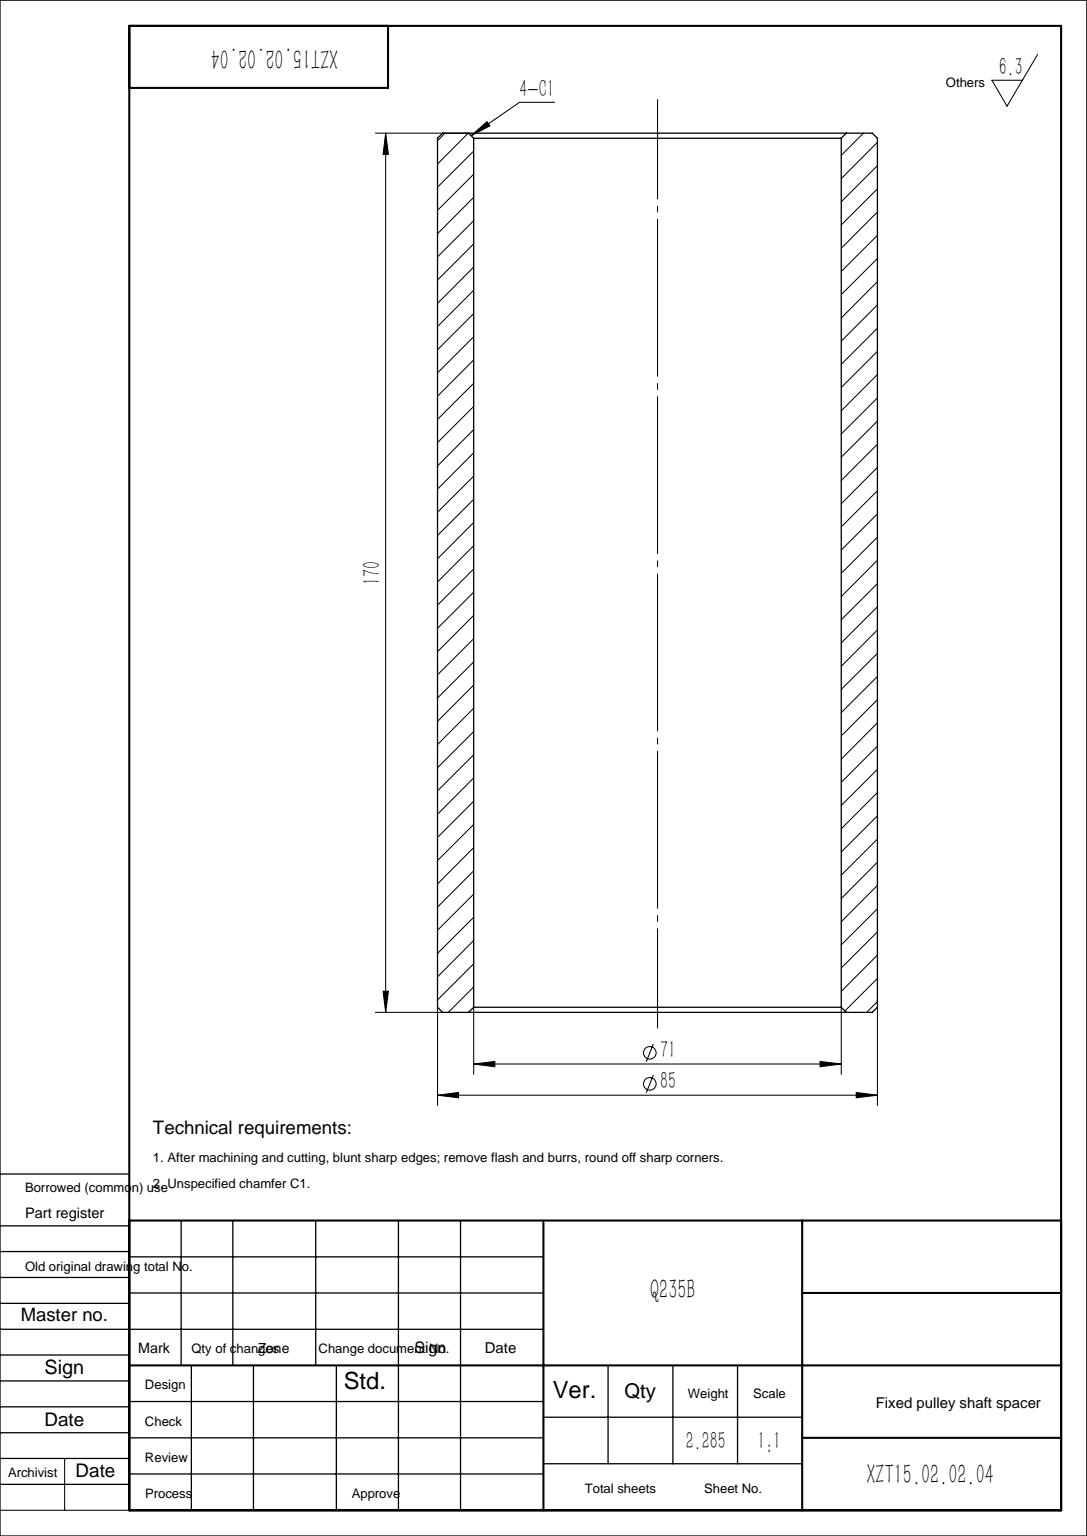
SolidWorks part; units mm, degrees
material "Q235B"
ref_plane "Front Plane" through (0, 0, 0) normal (0, 0, 1) x (1, 0, 0)
ref_plane "Top Plane" through (0, 0, 0) normal (0, 1, 0) x (1, 0, 0)
ref_plane "Right Plane" through (0, 0, 0) normal (1, 0, 0) x (0, 0, -1)
sketch "Sketch1" plane through (0, 0, 0) normal (0, 1, 0) x (1, 0, 0)
  circle A0 centre (0, 0) radius 35.5
  circle A1 centre (0, 0) radius 42.5
  dimension "D1" = 71
  dimension "D2" = 85
extrude "Boss-Extrude1" add sketch "Sketch1" along normal blind 170
chamfer "Chamfer2" distance 1 angle 45 4 edges at (0, 0, 35.5) (0, 170, 35.5) (0, 0, 42.5) (0, 170, 42.5)
